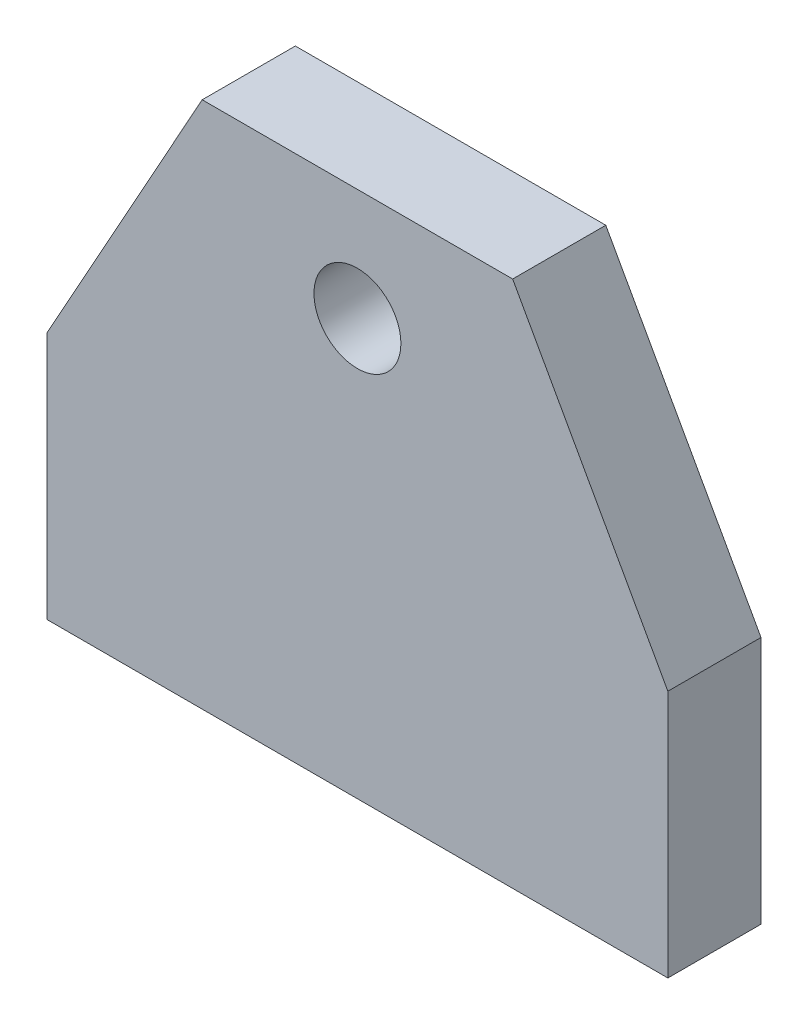
SolidWorks part; units mm, degrees
material "Q235-A"
ref_plane "Front Plane" through (0, 0, 0) normal (0, 0, 1) x (1, 0, 0)
ref_plane "Top Plane" through (0, 0, 0) normal (0, 1, 0) x (1, 0, 0)
ref_plane "Right Plane" through (0, 0, 0) normal (1, 0, 0) x (0, 0, -1)
sketch "Sketch1" plane through (0, 0, 0) normal (0, 0, 1) x (1, 0, 0)
  line L0 (0, 0) -> (0, 92.2651) construction
  line L1 (-50, 0) -> (50, 0)
  line L2 (50, 0) -> (50, 40)
  line L3 (50, 40) -> (25, 85)
  line L4 (25, 85) -> (-25, 85)
  line L5 (-50, 40) -> (-25, 85)
  line L6 (-50, 0) -> (-50, 40)
  point P8 (0, 85)
  dimension "D1" = 100
  dimension "D2" = 85
  dimension "D3" = 40
  dimension "D4" = 50
extrude "Boss-Extrude1" add sketch "Sketch1" along normal mid plane 15
sketch "Sketch2" plane through (0, 0, 7.5) normal (0, 0, 1) x (1, 0, 0)
  line L0 (0, 0) -> (0, 67) construction
  dimension "D1" = 67
hole_wizard "M16 Tapped Hole1" positions "3DSketch1" profile "Sketch3" tap size "M16" standard "GB" end condition through all
sketch3d "3DSketch1"
  point P0 (0, 67, 7.5)
sketch "Sketch3" plane through (0, 67, 7.5) normal (1, 0, 0) x (0, -1, 0)
  line L0 (0, 0) -> (0, 15)
  line L1 (0, 15) -> (7, 15)
  line L2 (7, 15) -> (7, 0)
  line L5 (7, 0) -> (0, 0)
  line L11 (0, -6.35) -> (0, 107.95) construction
  dimension "通孔螺纹孔钻头直径" = 14
  dimension "通孔螺纹孔钻头深度" = 15
cosmetic thread "hole cosmetic thread 1" parameters "D2"=16
